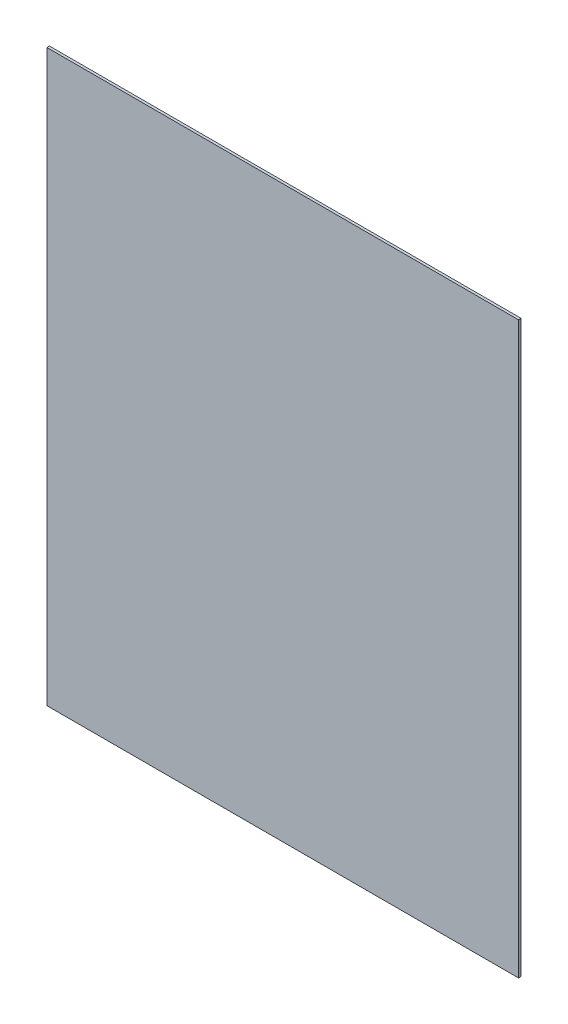
SolidWorks part; units mm, degrees
material "PMMA(有机玻璃)"
ref_plane "前视" through (0, 0, 0) normal (0, 0, 1) x (1, 0, 0)
ref_plane "上视" through (0, 0, 0) normal (0, 1, 0) x (1, 0, 0)
ref_plane "右视" through (0, 0, 0) normal (1, 0, 0) x (0, 0, -1)
sketch "草图1" plane through (0, 0, 0) normal (0, 0, 1) x (1, 0, 0)
  line L1 (-463, 559.5) -> (463, 559.5)
  line L2 (-463, 559.5) -> (-463, -559.5)
  line L3 (-463, -559.5) -> (463, -559.5)
  line L4 (463, 559.5) -> (463, -559.5)
  line L5 (-463, 559.5) -> (463, -559.5) construction
  line L6 (-463, -559.5) -> (463, 559.5) construction
  point P0 (0, 0)
  dimension "D1" = 1119
  dimension "D2" = 926
extrude "凸台-拉伸1" add sketch "草图1" along normal blind 5
